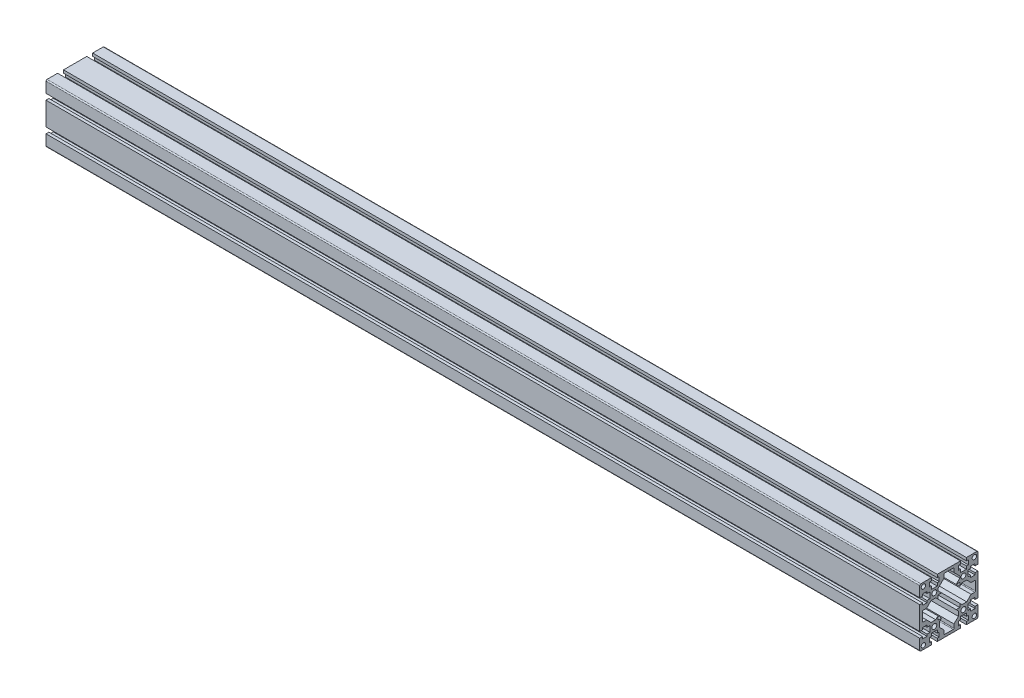
from build123d import *

# Parameters (mm, degrees)
SKETCH1_R                                 = 3.4
SKETCH1_R_2                               = 3
ALUMINIUM_PROFILE_80_X_80G_X_R1_5_1_DEPTH = 1200
SKETCH10_R                                = 3
CUT_EXTRUDE1_DEPTH                        = 1202.332593414


with BuildPart() as part:
    # Sketch1 → Aluminium profile 80 X 80G X R1.5(1) (new body)
    with BuildSketch(Plane.YZ.offset(-530.344827586)):
        with BuildLine():
            Line((-24.05, 40), (-24.05, 36))
            Line((-24.05, 36), (-26.75, 36))
            Line((-26.75, 36), (-26.75, 30))
            Line((-26.75, 30), (-24.05, 30))
            Line((-24.05, 30), (-24.05, 26))
            Line((-24.05, 26), (-15.95, 26))
            Line((-15.95, 26), (-15.95, 30))
            Line((-15.95, 30), (-13.25, 30))
            Line((-13.25, 30), (-13.25, 36))
            Line((-13.25, 36), (-15.95, 36))
            Line((-15.95, 36), (-15.95, 40))
            Line((-15.95, 40), (15.95, 40))
            Line((15.95, 40), (15.95, 36))
            Line((15.95, 36), (13.25, 36))
            Line((13.25, 36), (13.25, 30))
            Line((13.25, 30), (15.95, 30))
            Line((15.95, 30), (15.95, 26))
            Line((15.95, 26), (24.05, 26))
            Line((24.05, 26), (24.05, 30))
            Line((24.05, 30), (26.75, 30))
            Line((26.75, 30), (26.75, 36))
            Line((26.75, 36), (24.05, 36))
            Line((24.05, 36), (24.05, 40))
            Line((24.05, 40), (38.5, 40))
            ThreePointArc((38.5, 40), (39.560660172, 39.560660172), (40, 38.5))
            Line((40, 38.5), (40, 24.05))
            Line((40, 24.05), (36, 24.05))
            Line((36, 24.05), (36, 26.75))
            Line((36, 26.75), (30, 26.75))
            Line((30, 26.75), (30, 24.05))
            Line((30, 24.05), (26, 24.05))
            Line((26, 24.05), (26, 15.95))
            Line((26, 15.95), (30, 15.95))
            Line((30, 15.95), (30, 13.25))
            Line((30, 13.25), (36, 13.25))
            Line((36, 13.25), (36, 15.95))
            Line((36, 15.95), (40, 15.95))
            Line((40, 15.95), (40, -15.95))
            Line((40, -15.95), (36, -15.95))
            Line((36, -15.95), (36, -13.25))
            Line((36, -13.25), (30, -13.25))
            Line((30, -13.25), (30, -15.95))
            Line((30, -15.95), (26, -15.95))
            Line((26, -15.95), (26, -24.05))
            Line((26, -24.05), (30, -24.05))
            Line((30, -24.05), (30, -26.75))
            Line((30, -26.75), (36, -26.75))
            Line((36, -26.75), (36, -24.05))
            Line((36, -24.05), (40, -24.05))
            Line((40, -24.05), (40, -38.5))
            ThreePointArc((40, -38.5), (39.560660172, -39.560660172), (38.5, -40))
            Line((38.5, -40), (24.05, -40))
            Line((24.05, -40), (24.05, -36))
            Line((24.05, -36), (26.75, -36))
            Line((26.75, -36), (26.75, -30))
            Line((26.75, -30), (24.05, -30))
            Line((24.05, -30), (24.05, -26))
            Line((24.05, -26), (15.95, -26))
            Line((15.95, -26), (15.95, -30))
            Line((15.95, -30), (13.25, -30))
            Line((13.25, -30), (13.25, -36))
            Line((13.25, -36), (15.95, -36))
            Line((15.95, -36), (15.95, -40))
            Line((15.95, -40), (-15.95, -40))
            Line((-15.95, -40), (-15.95, -36))
            Line((-15.95, -36), (-13.25, -36))
            Line((-13.25, -36), (-13.25, -30))
            Line((-13.25, -30), (-15.95, -30))
            Line((-15.95, -30), (-15.95, -26))
            Line((-15.95, -26), (-24.05, -26))
            Line((-24.05, -26), (-24.05, -30))
            Line((-24.05, -30), (-26.75, -30))
            Line((-26.75, -30), (-26.75, -36))
            Line((-26.75, -36), (-24.05, -36))
            Line((-24.05, -36), (-24.05, -40))
            Line((-24.05, -40), (-38.5, -40))
            ThreePointArc((-38.5, -40), (-39.560660172, -39.560660172), (-40, -38.5))
            Line((-40, -38.5), (-40, -24.05))
            Line((-40, -24.05), (-36, -24.05))
            Line((-36, -24.05), (-36, -26.75))
            Line((-36, -26.75), (-30, -26.75))
            Line((-30, -26.75), (-30, -24.05))
            Line((-30, -24.05), (-26, -24.05))
            Line((-26, -24.05), (-26, -15.95))
            Line((-26, -15.95), (-30, -15.95))
            Line((-30, -15.95), (-30, -13.25))
            Line((-30, -13.25), (-36, -13.25))
            Line((-36, -13.25), (-36, -15.95))
            Line((-36, -15.95), (-40, -15.95))
            Line((-40, -15.95), (-40, 15.95))
            Line((-40, 15.95), (-36, 15.95))
            Line((-36, 15.95), (-36, 13.25))
            Line((-36, 13.25), (-30, 13.25))
            Line((-30, 13.25), (-30, 15.95))
            Line((-30, 15.95), (-26, 15.95))
            Line((-26, 15.95), (-26, 24.05))
            Line((-26, 24.05), (-30, 24.05))
            Line((-30, 24.05), (-30, 26.75))
            Line((-30, 26.75), (-36, 26.75))
            Line((-36, 26.75), (-36, 24.05))
            Line((-36, 24.05), (-40, 24.05))
            Line((-40, 24.05), (-40, 38.5))
            ThreePointArc((-40, 38.5), (-39.560660172, 39.560660172), (-38.5, 40))
            Line((-38.5, 40), (-24.05, 40))
        make_face()
        with Locations((-20, 20)):
            Circle(SKETCH1_R, mode=Mode.SUBTRACT)
        with Locations((20, 20)):
            Circle(SKETCH1_R, mode=Mode.SUBTRACT)
        with Locations((20, -20)):
            Circle(SKETCH1_R, mode=Mode.SUBTRACT)
        with Locations((-20, -20)):
            Circle(SKETCH1_R, mode=Mode.SUBTRACT)
        with Locations((-35, 35)):
            Circle(SKETCH1_R_2, mode=Mode.SUBTRACT)
        with Locations((35, 35)):
            Circle(SKETCH1_R_2, mode=Mode.SUBTRACT)
        with Locations((35, -35)):
            Circle(SKETCH1_R_2, mode=Mode.SUBTRACT)
        with BuildLine():
            Line((-13, 18), (-10, 15))
            Line((-10, 15), (-15, 15))
            Line((-15, 15), (-15, 10))
            Line((-15, 10), (-18, 13))
            Line((-18, 13), (-24.5, 13))
            Line((-24.5, 13), (-30.5, 7))
            Line((-30.5, 7), (-35.5, 7))
            ThreePointArc((-35.5, 7), (-36.207106781, 6.707106781), (-36.5, 6))
            Line((-36.5, 6), (-36.5, -6))
            ThreePointArc((-36.5, -6), (-36.207106781, -6.707106781), (-35.5, -7))
            Line((-35.5, -7), (-30.5, -7))
            Line((-30.5, -7), (-24.5, -13))
            Line((-24.5, -13), (-18, -13))
            Line((-18, -13), (-15, -10))
            Line((-15, -10), (-15, -15))
            Line((-15, -15), (-10, -15))
            Line((-10, -15), (-13, -18))
            Line((-13, -18), (-13, -24.5))
            Line((-13, -24.5), (-7, -30.5))
            Line((-7, -30.5), (-7, -35.5))
            ThreePointArc((-7, -35.5), (-6.707106781, -36.207106781), (-6, -36.5))
            Line((-6, -36.5), (6, -36.5))
            ThreePointArc((6, -36.5), (6.707106781, -36.207106781), (7, -35.5))
            Line((7, -35.5), (7, -30.5))
            Line((7, -30.5), (13, -24.5))
            Line((13, -24.5), (13, -18))
            Line((13, -18), (10, -15))
            Line((10, -15), (15, -15))
            Line((15, -15), (15, -10))
            Line((15, -10), (20, -15))
            Line((20, -15), (22.5, -15))
            Line((22.5, -15), (30.5, -7))
            Line((30.5, -7), (35.5, -7))
            ThreePointArc((35.5, -7), (36.207106781, -6.707106781), (36.5, -6))
            Line((36.5, -6), (36.5, 6))
            ThreePointArc((36.5, 6), (36.207106781, 6.707106781), (35.5, 7))
            Line((35.5, 7), (30.5, 7))
            Line((30.5, 7), (22.5, 15))
            Line((22.5, 15), (20, 15))
            Line((20, 15), (15, 10))
            Line((15, 10), (15, 15))
            Line((15, 15), (10, 15))
            Line((10, 15), (13, 18))
            Line((13, 18), (13, 24.5))
            Line((13, 24.5), (7, 30.5))
            Line((7, 30.5), (7, 35.5))
            ThreePointArc((7, 35.5), (6.707106781, 36.207106781), (6, 36.5))
            Line((6, 36.5), (-6, 36.5))
            ThreePointArc((-6, 36.5), (-6.707106781, 36.207106781), (-7, 35.5))
            Line((-7, 35.5), (-7, 30.5))
            Line((-7, 30.5), (-13, 24.5))
            Line((-13, 24.5), (-13, 18))
        make_face(mode=Mode.SUBTRACT)
    extrude(amount=ALUMINIUM_PROFILE_80_X_80G_X_R1_5_1_DEPTH)

    # Sketch10 → Cut-Extrude1 (cut, through all)
    with BuildSketch(Plane(origin=(669.655172414, 0, 0), x_dir=(0, 0, -1), z_dir=(1, 0, 0))):
        with Locations((35, -35)):
            Circle(SKETCH10_R)
    extrude(amount=-CUT_EXTRUDE1_DEPTH, mode=Mode.SUBTRACT)


solid = part.part
